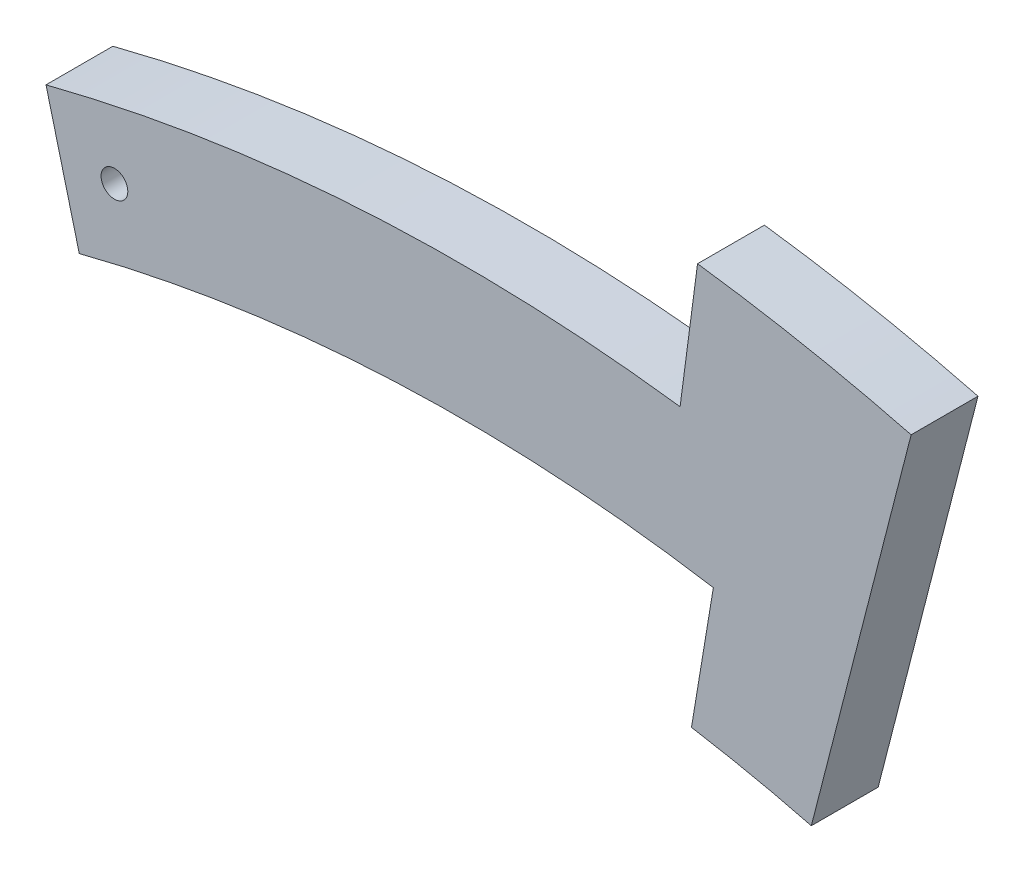
from build123d import *

# Parameters (mm, degrees)
BOSS_EXTRUDE3_DEPTH = 5
SKETCH3_R           = 1
CUT_EXTRUDE1_DEPTH  = 10


with BuildPart() as part:
    # Sketch1 → Boss-Extrude3 (new body)
    with BuildSketch(Plane.XY):
        with BuildLine():
            Line((26.130187968, 101.696672889), (28.618777298, 111.382070307))
            Line((28.618777298, 111.382070307), (31.107366629, 121.067467725))
            Line((31.107366629, 121.067467725), (33.595955959, 130.752865143))
            ThreePointArc((33.595955959, 130.752865143), (27.860620179, 132.093852405), (22.072250126, 133.183391511))
            ThreePointArc((22.072250126, 133.183391511), (19.849400241, 133.53277242), (17.62103595, 133.845056285))
            Line((17.62103595, 133.845056285), (16.315774028, 123.930607672))
            ThreePointArc((16.315774028, 123.930607672), (-7.533073444, 124.772804747), (-31.107366629, 121.067467725))
            Line((-31.107366629, 121.067467725), (-28.618777298, 111.382070307))
            ThreePointArc((-28.618777298, 111.382070307), (-5.016229547, 114.890545482), (18.802287144, 113.452518695))
            Line((18.802287144, 113.452518695), (17.167305653, 103.587082286))
            ThreePointArc((17.167305653, 103.587082286), (21.669371251, 102.739662982), (26.130187968, 101.696672889))
        make_face()
    extrude(amount=BOSS_EXTRUDE3_DEPTH)

    # Sketch3 → Cut-Extrude1 (cut)
    with BuildSketch(Plane(origin=(0, 0, 0), x_dir=(-1, 0, 0), z_dir=(0, 0, -1))):
        with Locations((25.988912996, 117.220204748)):
            Circle(SKETCH3_R)
    extrude(amount=-CUT_EXTRUDE1_DEPTH, mode=Mode.SUBTRACT)


solid = part.part
